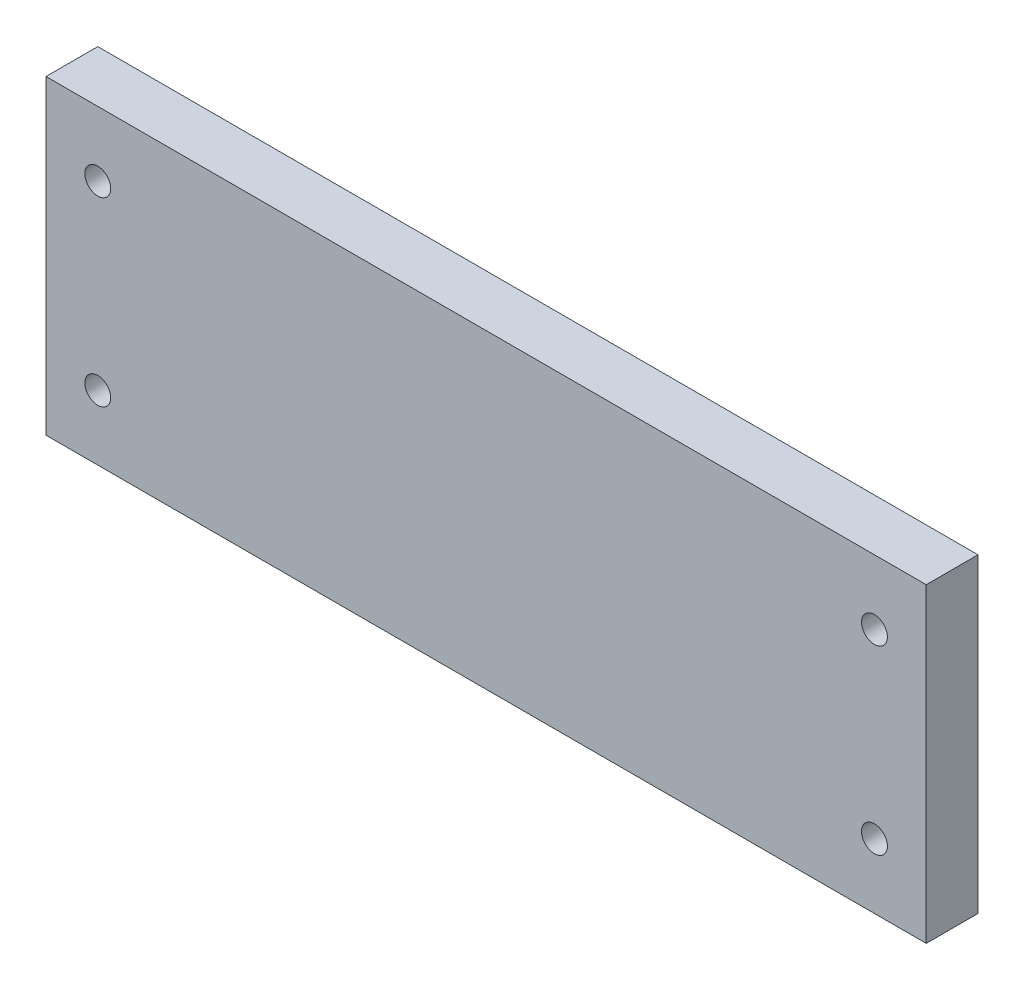
SolidWorks part; units mm, degrees
material "Q235B"
ref_plane "Front Plane" through (0, 0, 0) normal (0, 0, 1) x (1, 0, 0)
ref_plane "Top Plane" through (0, 0, 0) normal (0, 1, 0) x (1, 0, 0)
ref_plane "Right Plane" through (0, 0, 0) normal (1, 0, 0) x (0, 0, -1)
sketch "Sketch1" plane through (0, 0, 0) normal (0, 0, 1) x (1, 0, 0)
  line L1 (0, 0) -> (340, 0)
  line L2 (0, 0) -> (0, 120)
  line L3 (0, 120) -> (340, 120)
  line L4 (340, 0) -> (340, 120)
  circle A0 centre (20, 95) radius 5
  circle A1 centre (320, 95) radius 5
  circle A2 centre (320, 25) radius 5
  circle A3 centre (20, 25) radius 5
  dimension "D5" = 25
  dimension "D6" = 70
  dimension "D7" = 300
  dimension "D3" = 10
  dimension "D4" = 20
  dimension "D1" = 340
  dimension "D2" = 120
extrude "Boss-Extrude1" add sketch "Sketch1" along normal blind 20
